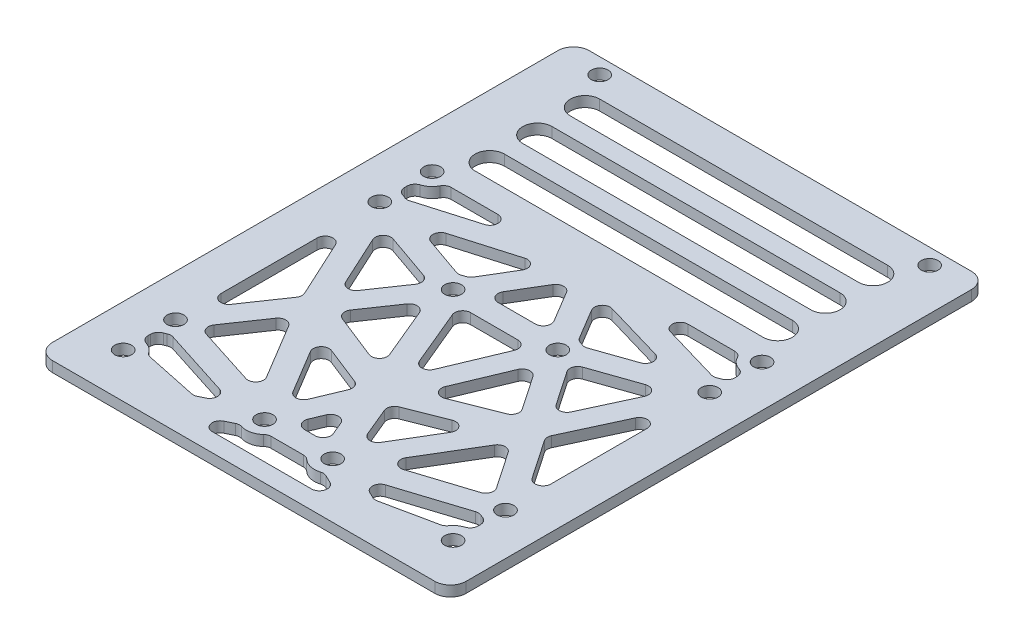
SolidWorks part; units mm, degrees
material "Thornel Mat VMA"
ref_plane "前视基准面" through (0, 0, 0) normal (0, 0, 1) x (1, 0, 0)
ref_plane "上视基准面" through (0, 0, 0) normal (0, 1, 0) x (1, 0, 0)
ref_plane "右视基准面" through (0, 0, 0) normal (1, 0, 0) x (0, 0, -1)
sketch "草图1" plane through (0, 0, 0) normal (0, 1, 0) x (1, 0, 0)
  line L0 (0, 56) -> (0, -46.5) construction
  line L1 (-39.5, 56) -> (39.5, 56)
  line L2 (-39.5, 56) -> (-39.5, -46.5)
  line L3 (-39.5, -46.5) -> (39.5, -46.5)
  line L4 (39.5, 56) -> (39.5, -46.5)
  line L5 (-31.5, 21) -> (-31.5, 11) construction
  line L6 (31.5, 21) -> (31.5, 11) construction
  line L7 (-10, 3.5) -> (10, 3.5) construction
  line L8 (-6.5, -36) -> (6.5, -36) construction
  line L9 (-31.5, -28) -> (-31.5, -38) construction
  line L10 (31.5, -28) -> (31.5, -38) construction
  circle A0 centre (-31.5, 11) radius 1.6
  circle A1 centre (-31.5, 21) radius 1.6
  circle A2 centre (31.5, 11) radius 1.6
  circle A3 centre (31.5, 21) radius 1.6
  circle A4 centre (-6.5, -36) radius 1.6
  circle A5 centre (6.5, -36) radius 1.6
  circle A6 centre (-10, 3.5) radius 1.6
  circle A7 centre (10, 3.5) radius 1.6
  circle A8 centre (-31.5, 53) radius 1.6
  circle A9 centre (31.5, 53) radius 1.6
  circle A10 centre (-31.5, -28) radius 1.6
  circle A11 centre (-31.5, -38) radius 1.6
  circle A12 centre (31.5, -38) radius 1.6
  circle A13 centre (31.5, -28) radius 1.6
  point P37 (-118.0265, 42.8023)
  dimension "D2" = 8
  dimension "D3" = 3.2
  dimension "D5" = 20
  dimension "D12" = 3
  dimension "D13" = 2
  dimension "D1" = 79
  dimension "D4" = 10
  dimension "D6" = 3.5
  dimension "D7" = 52.5
  dimension "D8" = 46.5
  dimension "D9" = 13
  dimension "D10" = 10.5
  dimension "D11" = 11
  dimension "D14" = 28
extrude "凸台-拉伸1" add sketch "草图1" along normal blind 2
sketch "草图2" plane through (0, 2, 0) normal (0, 1, 0) x (1, 0, 0)
  line L0 (0, 56) -> (0, -46.5) construction
  line L1 (39.5, 56) -> (-39.5, 56) construction
  line L2 (-39.5, -46.5) -> (39.5, -46.5) construction
  line L3 (-27.5, 46.2) -> (27.5, 46.2) construction
  line L4 (-27.5, 49) -> (27.5, 49)
  line L5 (-27.5, 43.4) -> (27.5, 43.4)
  line L6 (-39.5, 56) -> (-39.5, -46.5) construction
  line L7 (-27.5, 37.1) -> (27.5, 37.1) construction
  line L8 (-27.5, 39.9) -> (27.5, 39.9)
  line L9 (-27.5, 34.3) -> (27.5, 34.3)
  line L10 (-27.5, 28) -> (27.5, 28) construction
  line L11 (-27.5, 30.8) -> (27.5, 30.8)
  line L12 (-27.5, 25.2) -> (27.5, 25.2)
  line L13 (-31.5, -38) -> (-16.9387, -41.0657) construction
  line L16 (-16, -43) -> (16, -43)
  line L19 (-31.0571, -35.8961) -> (-16.4957, -38.9619)
  line L22 (-31.9429, -40.1039) -> (-17.3816, -43.1696)
  line L25 (-31.5, 11) -> (-10, 3.5) construction
  line L28 (-30.7918, 13.03) -> (-9.2918, 5.53)
  line L31 (-10, 3.5) -> (10, 3.5) construction
  line L32 (-10, 5.65) -> (10, 5.65)
  line L33 (-10, 1.35) -> (10, 1.35)
  line L37 (-32.2082, 8.97) -> (-10.7082, 1.47)
  line L43 (-16.9387, -41.0657) -> (-6.5, -36) construction
  line L44 (-17.8773, -39.1315) -> (-7.4387, -34.0657)
  line L45 (-16, -43) -> (-5.5613, -37.9343)
  line L46 (16.9387, -41.0657) -> (6.5, -36) construction
  line L49 (-31.5, -28) -> (-10, 3.5) construction
  line L56 (-33.2758, -26.788) -> (-11.7758, 4.712)
  line L59 (-29.7242, -29.212) -> (-8.2242, 2.288)
  line L62 (-31.5, 11) -> (-31.5, -28)
  line L65 (-31.5, -28) -> (-6.5, -36) construction
  line L68 (-6.5, -36) -> (6.5, -36) construction
  line L69 (-6.5, -33.85) -> (6.5, -33.85)
  line L70 (-6.5, -38.15) -> (6.5, -38.15)
  line L71 (-30.8447, -25.9523) -> (-5.8447, -33.9523)
  line L72 (-32.1553, -30.0477) -> (-7.1553, -38.0477)
  line L73 (-31.5, -28) -> (-31.5, -38)
  line L74 (17.8773, -39.1315) -> (7.4387, -34.0657)
  line L75 (16, -43) -> (5.5613, -37.9343)
  line L76 (-10, 3.5) -> (6.5, -36) construction
  line L77 (-8.0161, 4.3287) -> (8.4839, -35.1713)
  line L78 (-11.9839, 2.6713) -> (4.5161, -36.8287)
  line L79 (-6.5, -36) -> (10, 3.5) construction
  line L80 (-8.4839, -35.1713) -> (8.0161, 4.3287)
  line L81 (-4.5161, -36.8287) -> (11.9839, 2.6713)
  line L82 (-31.5, 11) -> (-20.75, -12.25) construction
  line L83 (-29.5485, 11.9023) -> (-18.7985, -11.3477)
  line L84 (-33.4515, 10.0977) -> (-22.7015, -13.1523)
  line L85 (-20.75, -12.25) -> (-6.5, -36) construction
  line L86 (-18.9064, -11.1438) -> (-4.6564, -34.8938)
  line L87 (-22.5936, -13.3562) -> (-8.3436, -37.1062)
  line L88 (-20.75, -12.25) -> (0, -20.4394) construction
  line L89 (-19.9607, -10.2501) -> (0.7893, -18.4395)
  line L90 (-21.5393, -14.2499) -> (-0.7893, -22.4393)
  line L91 (-28.0927, 20.2) -> (28.0927, 20.2)
  line L92 (-31.5, 17.5) -> (-31.5, 14.5)
  line L93 (31.5, 17.5) -> (31.5, 14.5)
  line L94 (-31.5, 11) -> (0, 20.2) construction
  line L95 (-32.1028, 13.0638) -> (-0.6028, 22.2638)
  line L96 (-30.8972, 8.9362) -> (0.6028, 18.1362)
  line L97 (-10, 3.5) -> (0, 20.2) construction
  line L98 (-11.8446, 4.6045) -> (-1.8446, 21.3045)
  line L99 (-8.1554, 2.3955) -> (1.8446, 19.0955)
  line L100 (31.5, -28) -> (31.5, -38)
  line L101 (31.5, 11) -> (31.5, -28)
  line L102 (31.5, -38) -> (16.9387, -41.0657) construction
  line L103 (31.0571, -35.8961) -> (16.4957, -38.9619)
  line L104 (31.9429, -40.1039) -> (17.3816, -43.1696)
  line L105 (31.5, -28) -> (6.5, -36) construction
  line L106 (30.8447, -25.9523) -> (5.8447, -33.9523)
  line L107 (32.1553, -30.0477) -> (7.1553, -38.0477)
  line L108 (20.75, -12.25) -> (0, -20.4394) construction
  line L109 (19.9607, -10.2501) -> (-0.7893, -18.4395)
  line L110 (21.5393, -14.2499) -> (0.7893, -22.4393)
  line L111 (20.75, -12.25) -> (6.5, -36) construction
  line L112 (18.9064, -11.1438) -> (4.6564, -34.8938)
  line L113 (22.5936, -13.3562) -> (8.3436, -37.1062)
  line L114 (31.5, -28) -> (10, 3.5) construction
  line L115 (33.2758, -26.788) -> (11.7758, 4.712)
  line L116 (29.7242, -29.212) -> (8.2242, 2.288)
  line L117 (31.5, 11) -> (20.75, -12.25) construction
  line L118 (29.5485, 11.9023) -> (18.7985, -11.3477)
  line L119 (33.4515, 10.0977) -> (22.7015, -13.1523)
  line L120 (31.5, 11) -> (10, 3.5) construction
  line L121 (30.7918, 13.03) -> (9.2918, 5.53)
  line L122 (32.2082, 8.97) -> (10.7082, 1.47)
  line L123 (10, 3.5) -> (0, 20.2) construction
  line L124 (11.8446, 4.6045) -> (1.8446, 21.3045)
  line L125 (8.1554, 2.3955) -> (-1.8446, 19.0955)
  line L126 (31.5, 11) -> (0, 20.2) construction
  line L127 (32.1028, 13.0638) -> (0.6028, 22.2638)
  line L128 (30.8972, 8.9362) -> (-0.6028, 18.1362)
  arc A0 (-27.5, 49) -> (-27.5, 43.4) centre (-27.5, 46.2) ccw
  arc A1 (27.5, 43.4) -> (27.5, 49) centre (27.5, 46.2) ccw
  arc A2 (-27.5, 39.9) -> (-27.5, 34.3) centre (-27.5, 37.1) ccw
  arc A3 (27.5, 34.3) -> (27.5, 39.9) centre (27.5, 37.1) ccw
  arc A4 (-27.5, 30.8) -> (-27.5, 25.2) centre (-27.5, 28) ccw
  arc A5 (27.5, 25.2) -> (27.5, 30.8) centre (27.5, 28) ccw
  arc A18 (-10, 5.65) -> (-10, 1.35) centre (-10, 3.5) ccw
  arc A19 (10, 1.35) -> (10, 5.65) centre (10, 3.5) ccw
  arc A26 (-17.8773, -39.1315) -> (-16, -43) centre (-16.9387, -41.0657) ccw
  arc A27 (-5.5613, -37.9343) -> (-7.4387, -34.0657) centre (-6.5, -36) ccw
  circle A44 centre (-10, 3.5) radius 3.5
  circle A45 centre (-31.5, 11) radius 3.5
  circle A46 centre (-6.5, -36) radius 3.5
  circle A48 centre (10, 3.5) radius 3.5
  circle A49 centre (31.5, 11) radius 3.5
  circle A50 centre (6.5, -36) radius 3.5
  arc A54 (-6.5, -33.85) -> (-6.5, -38.15) centre (-6.5, -36) ccw
  arc A55 (6.5, -38.15) -> (6.5, -33.85) centre (6.5, -36) ccw
  circle A56 centre (-31.5, -28) radius 3.5
  circle A57 centre (-31.5, -38) radius 3.5
  circle A58 centre (31.5, -28) radius 3.5
  circle A59 centre (31.5, -38) radius 3.5
  arc A60 (-31.0571, -35.8961) -> (-31.9429, -40.1039) centre (-31.5, -38) ccw
  arc A61 (-17.3816, -43.1696) -> (-16.4957, -38.9619) centre (-16.9387, -41.0657) ccw
  arc A62 (-30.7918, 13.03) -> (-32.2082, 8.97) centre (-31.5, 11) ccw
  arc A63 (-10.7082, 1.47) -> (-9.2918, 5.53) centre (-10, 3.5) ccw
  arc A64 (-33.2758, -26.788) -> (-29.7242, -29.212) centre (-31.5, -28) ccw
  arc A65 (-8.2242, 2.288) -> (-11.7758, 4.712) centre (-10, 3.5) ccw
  arc A66 (-30.8447, -25.9523) -> (-32.1553, -30.0477) centre (-31.5, -28) ccw
  arc A67 (-7.1553, -38.0477) -> (-5.8447, -33.9523) centre (-6.5, -36) ccw
  arc A68 (17.8773, -39.1315) -> (16, -43) centre (16.9387, -41.0657) cw
  arc A69 (5.5613, -37.9343) -> (7.4387, -34.0657) centre (6.5, -36) cw
  arc A70 (-8.0161, 4.3287) -> (-11.9839, 2.6713) centre (-10, 3.5) ccw
  arc A71 (4.5161, -36.8287) -> (8.4839, -35.1713) centre (6.5, -36) ccw
  arc A72 (-8.4839, -35.1713) -> (-4.5161, -36.8287) centre (-6.5, -36) ccw
  arc A73 (11.9839, 2.6713) -> (8.0161, 4.3287) centre (10, 3.5) ccw
  arc A74 (-29.5485, 11.9023) -> (-33.4515, 10.0977) centre (-31.5, 11) ccw
  arc A75 (-22.7015, -13.1523) -> (-18.7985, -11.3477) centre (-20.75, -12.25) ccw
  arc A76 (-18.9064, -11.1438) -> (-22.5936, -13.3562) centre (-20.75, -12.25) ccw
  arc A77 (-8.3436, -37.1062) -> (-4.6564, -34.8938) centre (-6.5, -36) ccw
  arc A78 (-19.9607, -10.2501) -> (-21.5393, -14.2499) centre (-20.75, -12.25) ccw
  arc A79 (-0.7893, -22.4393) -> (0.7893, -18.4395) centre (0, -20.4394) ccw
  circle A80 centre (-31.5, 21) radius 3.5
  circle A81 centre (31.5, 21) radius 3.5
  arc A82 (-32.1028, 13.0638) -> (-30.8972, 8.9362) centre (-31.5, 11) ccw
  arc A83 (0.6028, 18.1362) -> (-0.6028, 22.2638) centre (0, 20.2) ccw
  arc A84 (-11.8446, 4.6045) -> (-8.1554, 2.3955) centre (-10, 3.5) ccw
  arc A85 (1.8446, 19.0955) -> (-1.8446, 21.3045) centre (0, 20.2) ccw
  arc A86 (31.0571, -35.8961) -> (31.9429, -40.1039) centre (31.5, -38) cw
  arc A87 (17.3816, -43.1696) -> (16.4957, -38.9619) centre (16.9387, -41.0657) cw
  arc A88 (30.8447, -25.9523) -> (32.1553, -30.0477) centre (31.5, -28) cw
  arc A89 (7.1553, -38.0477) -> (5.8447, -33.9523) centre (6.5, -36) cw
  arc A90 (19.9607, -10.2501) -> (21.5393, -14.2499) centre (20.75, -12.25) cw
  arc A91 (0.7893, -22.4393) -> (-0.7893, -18.4395) centre (0, -20.4394) cw
  arc A92 (18.9064, -11.1438) -> (22.5936, -13.3562) centre (20.75, -12.25) cw
  arc A93 (8.3436, -37.1062) -> (4.6564, -34.8938) centre (6.5, -36) cw
  arc A94 (33.2758, -26.788) -> (29.7242, -29.212) centre (31.5, -28) cw
  arc A95 (8.2242, 2.288) -> (11.7758, 4.712) centre (10, 3.5) cw
  arc A96 (29.5485, 11.9023) -> (33.4515, 10.0977) centre (31.5, 11) cw
  arc A97 (22.7015, -13.1523) -> (18.7985, -11.3477) centre (20.75, -12.25) cw
  arc A98 (30.7918, 13.03) -> (32.2082, 8.97) centre (31.5, 11) cw
  arc A99 (10.7082, 1.47) -> (9.2918, 5.53) centre (10, 3.5) cw
  arc A100 (11.8446, 4.6045) -> (8.1554, 2.3955) centre (10, 3.5) cw
  arc A101 (-1.8446, 19.0955) -> (1.8446, 21.3045) centre (0, 20.2) cw
  arc A102 (32.1028, 13.0638) -> (30.8972, 8.9362) centre (31.5, 11) cw
  arc A103 (-0.6028, 18.1362) -> (0.6028, 22.2638) centre (0, 20.2) cw
  point P8 (0, 46.2)
  point P18 (0, 37.1)
  point P25 (0, 28)
  point P37 (-24.2193, -39.5329)
  point P45 (0, -36)
  point P46 (-20.75, 7.25)
  point P51 (-20.75, -12.25)
  point P59 (-19, -32)
  point P68 (-1.75, -16.25)
  point P73 (11.7193, -38.5329)
  point P74 (0, 3.5)
  point P91 (1.75, -16.25)
  point P98 (-26.125, -0.625)
  point P105 (-11.7193, -38.5329)
  point P114 (-13.625, -24.125)
  point P119 (31.5, 11)
  point P120 (-10.375, -16.3447)
  point P144 (-31.5, 11)
  point P153 (-15.75, 15.6)
  point P158 (-5, 11.85)
  point P174 (24.2193, -39.5329)
  point P180 (19, -32)
  point P187 (10.375, -16.3447)
  point P194 (13.625, -24.125)
  point P201 (20.75, -12.25)
  point P207 (26.125, -0.625)
  point P214 (20.75, 7.25)
  point P221 (5, 11.85)
  point P228 (15.75, 15.6)
  point P233 (-16.2902, -41.2364)
  dimension "D1" = 2.8
  dimension "D10" = 7
  dimension "D7" = 4.3
  dimension "D8" = 5
  dimension "D2" = 7
  dimension "D3" = 12
  dimension "D5" = 3.5
  dimension "D6" = 3.5
  dimension "D9" = 32
  dimension "D4" = 3
extrude "切除-拉伸1" cut sketch "草图2" against normal through all contours L5 A1 L4 A0 | L9 A3 L8 A2 | L12 A5 L11 A4 | A80 L92 A45 L95 L91 | A81 L91 L127 A49 L93 | A44 L98 L96 L28 | L32 L125 L99 | L124 A48 L121 L128 | L37 L83 L56 | L59 L89 L78 | L77 L80 L33 | L84 L62 L56 | L118 L122 L115 | L109 L116 L81 | L101 L119 L115 | L87 L59 L71 | L90 L86 L80 | L81 L69 L78 | L112 L110 L77 | L106 L116 L113 | A57 L19 L44 L72 A56 L73 | L75 A50 L70 A46 L45 L16 | L103 A59 L100 A58 L107 L74
fillet "R1.5 镂空圆角" radius 1.5 75 edges at (-31.5, 1, 34.5) (-31.5, 1, 31.5) (-29.5249, 1, 30.8894) (-12.2709, 1, 36.4107) (-17.2155, 1, 38.8103) (-28.3545, 1, 36.4651) (0, 1, 26.0174) (3.2719, 1, 33.85) (-3.2719, 1, 33.85) (17.2155, 1, 38.8103) (12.2709, 1, 36.4107) (29.5249, 1, 30.8894) (31.5, 1, 31.5) (31.5, 1, 34.5) (28.3545, 1, 36.4651) (-16, 1, 43) (-8.046, 1, 39.14) (-3.7382, 1, 38.15) (3.7382, 1, 38.15) (8.046, 1, 39.14) (16, 1, 43) (0, 1, -16.015) (6.2066, 1, -5.65) (-6.2066, 1, -5.65) (4.6626, 1, -16.5984) (24.4523, 1, -10.8186) (11.8995, 1, -6.4397) (10.4257, 1, -6.974) (31.5, 1, -17.5) (31.5, 1, -14.5) (29.4517, 1, -13.8381) (7.669, 1, -20.2) (28.0927, 1, -20.2) (-11.2794, 1, 32.2132) (-28.099, 1, 26.8309) (-20.8666, 1, 16.2346) (31.5, 1, 24.1862) (23.2133, 1, 12.0453) (31.5, 1, -5.877) (-10.4572, 1, 0.9836) (-3.9461, 1, 16.5706) (-17.4565, 1, 11.2384) (20.3891, 1, 7.9075) (13.3578, 1, -2.3943) (27.4205, 1, -7.2999) (-23.2133, 1, 12.0453) (-31.5, 1, 24.1862) (-31.5, 1, -5.877) (6.7719, 1, -1.35) (0, 1, 14.8614) (-6.7719, 1, -1.35) (3.9461, 1, 16.5706) (10.4572, 1, 0.9836) (17.4565, 1, 11.2384) (-2.8291, 1, 21.6342) (-6.8446, 1, 31.2469) (-15.6476, 1, 16.5752) (-7.669, 1, -20.2) (-29.4517, 1, -13.8381) (-31.5, 1, -14.5) (-31.5, 1, -17.5) (-13.3578, 1, -2.3943) (-20.3891, 1, 7.9075) (-27.4205, 1, -7.2999) (-11.8995, 1, -6.4397) (-24.4523, 1, -10.8186) (-4.6626, 1, -16.5984) (-10.4257, 1, -6.974) (6.8446, 1, 31.2469) (2.8291, 1, 21.6342) (15.6476, 1, 16.5752) (11.2794, 1, 32.2132) (20.8666, 1, 16.2346) (28.099, 1, 26.8309) (-28.0927, 1, -20.2)
fillet "R3 外缘圆角" radius 3 4 edges at (-39.5, 1, -56) (39.5, 1, -56) (39.5, 1, 46.5) (-39.5, 1, 46.5)
